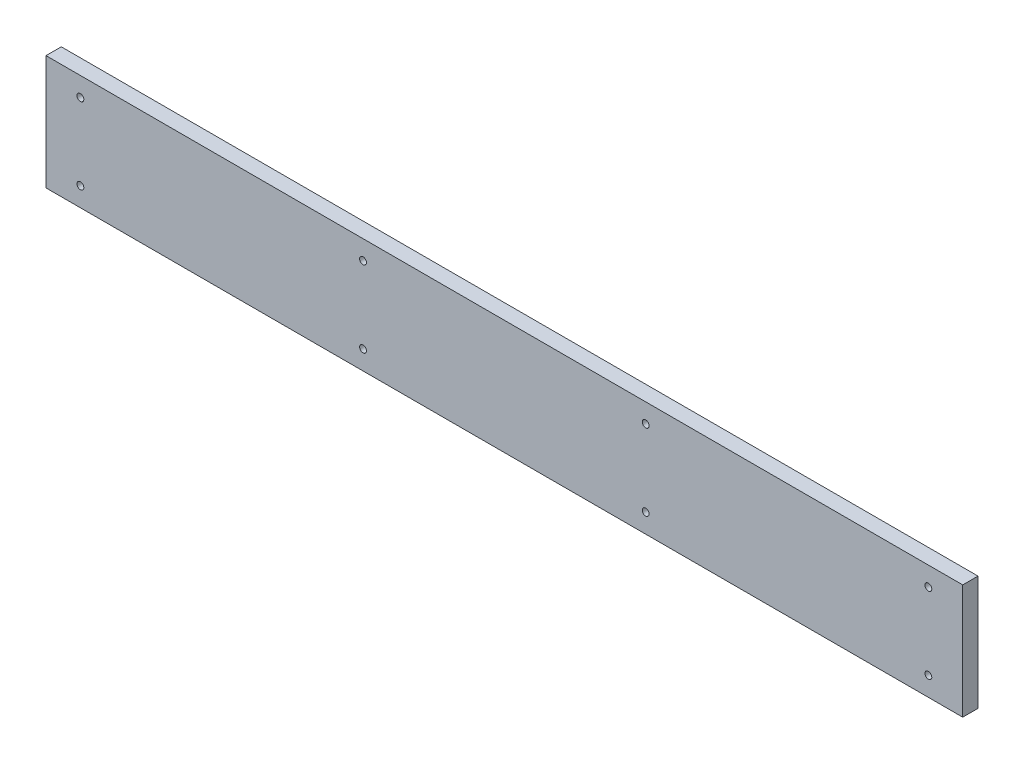
from build123d import *

# Parameters (mm, degrees)
SKETCH1_W                                           = 1200
SKETCH1_H                                           = 150
BOSS_EXTRUDE1_DEPTH                                 = 20
HOLE_SIZE_BY_SOCKET_HEAD_CAP_SCREW_TYPE_D           = 9
HOLE_SIZE_BY_SOCKET_HEAD_CAP_SCREW_TYPE_CBORE_D     = 15
HOLE_SIZE_BY_SOCKET_HEAD_CAP_SCREW_TYPE_CBORE_DEPTH = 9
SKETCH4_R                                           = 22.5
SKETCH4_R_2                                         = 19.5
CUT_EXTRUDE1_DEPTH                                  = 3
LPATTERN1_COUNT                                     = 4
LPATTERN1_PITCH                                     = 30
LPATTERN2_COUNT                                     = 23
LPATTERN2_PITCH                                     = 50
LPATTERN2_COPY_1_SKETCH_R                           = 22.5
LPATTERN2_COPY_1_SKETCH_R_2                         = 19.5
LPATTERN2_COPY_1_DEPTH                              = 3
LPATTERN2_COPY_2_SKETCH_R                           = 22.5
LPATTERN2_COPY_2_SKETCH_R_2                         = 19.5
LPATTERN2_COPY_2_DEPTH                              = 3
LPATTERN2_COPY_3_SKETCH_R                           = 22.5
LPATTERN2_COPY_3_SKETCH_R_2                         = 19.5
LPATTERN2_COPY_3_DEPTH                              = 3
LPATTERN2_COPY_4_SKETCH_R                           = 22.5
LPATTERN2_COPY_4_SKETCH_R_2                         = 19.5
LPATTERN2_COPY_4_DEPTH                              = 3
LPATTERN2_COPY_5_SKETCH_R                           = 22.5
LPATTERN2_COPY_5_SKETCH_R_2                         = 19.5
LPATTERN2_COPY_5_DEPTH                              = 3
LPATTERN2_COPY_6_SKETCH_R                           = 22.5
LPATTERN2_COPY_6_SKETCH_R_2                         = 19.5
LPATTERN2_COPY_6_DEPTH                              = 3
LPATTERN2_COPY_7_SKETCH_R                           = 22.5
LPATTERN2_COPY_7_SKETCH_R_2                         = 19.5
LPATTERN2_COPY_7_DEPTH                              = 3
LPATTERN2_COPY_8_SKETCH_R                           = 22.5
LPATTERN2_COPY_8_SKETCH_R_2                         = 19.5
LPATTERN2_COPY_8_DEPTH                              = 3
LPATTERN2_COPY_9_SKETCH_R                           = 22.5
LPATTERN2_COPY_9_SKETCH_R_2                         = 19.5
LPATTERN2_COPY_9_DEPTH                              = 3
LPATTERN2_COPY_10_SKETCH_R                          = 22.5
LPATTERN2_COPY_10_SKETCH_R_2                        = 19.5
LPATTERN2_COPY_10_DEPTH                             = 3
LPATTERN2_COPY_11_SKETCH_R                          = 22.5
LPATTERN2_COPY_11_SKETCH_R_2                        = 19.5
LPATTERN2_COPY_11_DEPTH                             = 3
LPATTERN2_COPY_12_SKETCH_R                          = 22.5
LPATTERN2_COPY_12_SKETCH_R_2                        = 19.5
LPATTERN2_COPY_12_DEPTH                             = 3
LPATTERN2_COPY_13_SKETCH_R                          = 22.5
LPATTERN2_COPY_13_SKETCH_R_2                        = 19.5
LPATTERN2_COPY_13_DEPTH                             = 3
LPATTERN2_COPY_14_SKETCH_R                          = 22.5
LPATTERN2_COPY_14_SKETCH_R_2                        = 19.5
LPATTERN2_COPY_14_DEPTH                             = 3
LPATTERN2_COPY_15_SKETCH_R                          = 22.5
LPATTERN2_COPY_15_SKETCH_R_2                        = 19.5
LPATTERN2_COPY_15_DEPTH                             = 3
LPATTERN2_COPY_16_SKETCH_R                          = 22.5
LPATTERN2_COPY_16_SKETCH_R_2                        = 19.5
LPATTERN2_COPY_16_DEPTH                             = 3
LPATTERN2_COPY_17_SKETCH_R                          = 22.5
LPATTERN2_COPY_17_SKETCH_R_2                        = 19.5
LPATTERN2_COPY_17_DEPTH                             = 3
LPATTERN2_COPY_18_SKETCH_R                          = 22.5
LPATTERN2_COPY_18_SKETCH_R_2                        = 19.5
LPATTERN2_COPY_18_DEPTH                             = 3
LPATTERN2_COPY_19_SKETCH_R                          = 22.5
LPATTERN2_COPY_19_SKETCH_R_2                        = 19.5
LPATTERN2_COPY_19_DEPTH                             = 3
LPATTERN2_COPY_20_SKETCH_R                          = 22.5
LPATTERN2_COPY_20_SKETCH_R_2                        = 19.5
LPATTERN2_COPY_20_DEPTH                             = 3
LPATTERN2_COPY_21_SKETCH_R                          = 22.5
LPATTERN2_COPY_21_SKETCH_R_2                        = 19.5
LPATTERN2_COPY_21_DEPTH                             = 3
LPATTERN2_COPY_22_SKETCH_R                          = 22.5
LPATTERN2_COPY_22_SKETCH_R_2                        = 19.5
LPATTERN2_COPY_22_DEPTH                             = 3
LPATTERN2_COPY_23_SKETCH_R                          = 22.5
LPATTERN2_COPY_23_SKETCH_R_2                        = 19.5
LPATTERN2_COPY_23_DEPTH                             = 3
LPATTERN2_COPY_24_SKETCH_R                          = 22.5
LPATTERN2_COPY_24_SKETCH_R_2                        = 19.5
LPATTERN2_COPY_24_DEPTH                             = 3
LPATTERN2_COPY_25_SKETCH_R                          = 22.5
LPATTERN2_COPY_25_SKETCH_R_2                        = 19.5
LPATTERN2_COPY_25_DEPTH                             = 3
LPATTERN2_COPY_26_SKETCH_R                          = 22.5
LPATTERN2_COPY_26_SKETCH_R_2                        = 19.5
LPATTERN2_COPY_26_DEPTH                             = 3
LPATTERN2_COPY_27_SKETCH_R                          = 22.5
LPATTERN2_COPY_27_SKETCH_R_2                        = 19.5
LPATTERN2_COPY_27_DEPTH                             = 3
LPATTERN2_COPY_28_SKETCH_R                          = 22.5
LPATTERN2_COPY_28_SKETCH_R_2                        = 19.5
LPATTERN2_COPY_28_DEPTH                             = 3
LPATTERN2_COPY_29_SKETCH_R                          = 22.5
LPATTERN2_COPY_29_SKETCH_R_2                        = 19.5
LPATTERN2_COPY_29_DEPTH                             = 3
LPATTERN2_COPY_30_SKETCH_R                          = 22.5
LPATTERN2_COPY_30_SKETCH_R_2                        = 19.5
LPATTERN2_COPY_30_DEPTH                             = 3
LPATTERN2_COPY_31_SKETCH_R                          = 22.5
LPATTERN2_COPY_31_SKETCH_R_2                        = 19.5
LPATTERN2_COPY_31_DEPTH                             = 3
LPATTERN2_COPY_32_SKETCH_R                          = 22.5
LPATTERN2_COPY_32_SKETCH_R_2                        = 19.5
LPATTERN2_COPY_32_DEPTH                             = 3
LPATTERN2_COPY_33_SKETCH_R                          = 22.5
LPATTERN2_COPY_33_SKETCH_R_2                        = 19.5
LPATTERN2_COPY_33_DEPTH                             = 3
LPATTERN2_COPY_34_SKETCH_R                          = 22.5
LPATTERN2_COPY_34_SKETCH_R_2                        = 19.5
LPATTERN2_COPY_34_DEPTH                             = 3
LPATTERN2_COPY_35_SKETCH_R                          = 22.5
LPATTERN2_COPY_35_SKETCH_R_2                        = 19.5
LPATTERN2_COPY_35_DEPTH                             = 3
LPATTERN2_COPY_36_SKETCH_R                          = 22.5
LPATTERN2_COPY_36_SKETCH_R_2                        = 19.5
LPATTERN2_COPY_36_DEPTH                             = 3
LPATTERN2_COPY_37_SKETCH_R                          = 22.5
LPATTERN2_COPY_37_SKETCH_R_2                        = 19.5
LPATTERN2_COPY_37_DEPTH                             = 3
LPATTERN2_COPY_38_SKETCH_R                          = 22.5
LPATTERN2_COPY_38_SKETCH_R_2                        = 19.5
LPATTERN2_COPY_38_DEPTH                             = 3
LPATTERN2_COPY_39_SKETCH_R                          = 22.5
LPATTERN2_COPY_39_SKETCH_R_2                        = 19.5
LPATTERN2_COPY_39_DEPTH                             = 3
LPATTERN2_COPY_40_SKETCH_R                          = 22.5
LPATTERN2_COPY_40_SKETCH_R_2                        = 19.5
LPATTERN2_COPY_40_DEPTH                             = 3
LPATTERN2_COPY_41_SKETCH_R                          = 22.5
LPATTERN2_COPY_41_SKETCH_R_2                        = 19.5
LPATTERN2_COPY_41_DEPTH                             = 3
LPATTERN2_COPY_42_SKETCH_R                          = 22.5
LPATTERN2_COPY_42_SKETCH_R_2                        = 19.5
LPATTERN2_COPY_42_DEPTH                             = 3
LPATTERN2_COPY_43_SKETCH_R                          = 22.5
LPATTERN2_COPY_43_SKETCH_R_2                        = 19.5
LPATTERN2_COPY_43_DEPTH                             = 3
LPATTERN2_COPY_44_SKETCH_R                          = 22.5
LPATTERN2_COPY_44_SKETCH_R_2                        = 19.5
LPATTERN2_COPY_44_DEPTH                             = 3
LPATTERN2_COPY_45_SKETCH_R                          = 22.5
LPATTERN2_COPY_45_SKETCH_R_2                        = 19.5
LPATTERN2_COPY_45_DEPTH                             = 3
LPATTERN2_COPY_46_SKETCH_R                          = 22.5
LPATTERN2_COPY_46_SKETCH_R_2                        = 19.5
LPATTERN2_COPY_46_DEPTH                             = 3
LPATTERN2_COPY_47_SKETCH_R                          = 22.5
LPATTERN2_COPY_47_SKETCH_R_2                        = 19.5
LPATTERN2_COPY_47_DEPTH                             = 3
LPATTERN2_COPY_48_SKETCH_R                          = 22.5
LPATTERN2_COPY_48_SKETCH_R_2                        = 19.5
LPATTERN2_COPY_48_DEPTH                             = 3
LPATTERN2_COPY_49_SKETCH_R                          = 22.5
LPATTERN2_COPY_49_SKETCH_R_2                        = 19.5
LPATTERN2_COPY_49_DEPTH                             = 3
LPATTERN2_COPY_50_SKETCH_R                          = 22.5
LPATTERN2_COPY_50_SKETCH_R_2                        = 19.5
LPATTERN2_COPY_50_DEPTH                             = 3
LPATTERN2_COPY_51_SKETCH_R                          = 22.5
LPATTERN2_COPY_51_SKETCH_R_2                        = 19.5
LPATTERN2_COPY_51_DEPTH                             = 3
LPATTERN2_COPY_52_SKETCH_R                          = 22.5
LPATTERN2_COPY_52_SKETCH_R_2                        = 19.5
LPATTERN2_COPY_52_DEPTH                             = 3
LPATTERN2_COPY_53_SKETCH_R                          = 22.5
LPATTERN2_COPY_53_SKETCH_R_2                        = 19.5
LPATTERN2_COPY_53_DEPTH                             = 3
LPATTERN2_COPY_54_SKETCH_R                          = 22.5
LPATTERN2_COPY_54_SKETCH_R_2                        = 19.5
LPATTERN2_COPY_54_DEPTH                             = 3
LPATTERN2_COPY_55_SKETCH_R                          = 22.5
LPATTERN2_COPY_55_SKETCH_R_2                        = 19.5
LPATTERN2_COPY_55_DEPTH                             = 3
LPATTERN2_COPY_56_SKETCH_R                          = 22.5
LPATTERN2_COPY_56_SKETCH_R_2                        = 19.5
LPATTERN2_COPY_56_DEPTH                             = 3
LPATTERN2_COPY_57_SKETCH_R                          = 22.5
LPATTERN2_COPY_57_SKETCH_R_2                        = 19.5
LPATTERN2_COPY_57_DEPTH                             = 3
LPATTERN2_COPY_58_SKETCH_R                          = 22.5
LPATTERN2_COPY_58_SKETCH_R_2                        = 19.5
LPATTERN2_COPY_58_DEPTH                             = 3
LPATTERN2_COPY_59_SKETCH_R                          = 22.5
LPATTERN2_COPY_59_SKETCH_R_2                        = 19.5
LPATTERN2_COPY_59_DEPTH                             = 3
LPATTERN2_COPY_60_SKETCH_R                          = 22.5
LPATTERN2_COPY_60_SKETCH_R_2                        = 19.5
LPATTERN2_COPY_60_DEPTH                             = 3
LPATTERN2_COPY_61_SKETCH_R                          = 22.5
LPATTERN2_COPY_61_SKETCH_R_2                        = 19.5
LPATTERN2_COPY_61_DEPTH                             = 3
LPATTERN2_COPY_62_SKETCH_R                          = 22.5
LPATTERN2_COPY_62_SKETCH_R_2                        = 19.5
LPATTERN2_COPY_62_DEPTH                             = 3
LPATTERN2_COPY_63_SKETCH_R                          = 22.5
LPATTERN2_COPY_63_SKETCH_R_2                        = 19.5
LPATTERN2_COPY_63_DEPTH                             = 3
LPATTERN2_COPY_64_SKETCH_R                          = 22.5
LPATTERN2_COPY_64_SKETCH_R_2                        = 19.5
LPATTERN2_COPY_64_DEPTH                             = 3
LPATTERN2_COPY_65_SKETCH_R                          = 22.5
LPATTERN2_COPY_65_SKETCH_R_2                        = 19.5
LPATTERN2_COPY_65_DEPTH                             = 3
LPATTERN2_COPY_66_SKETCH_R                          = 22.5
LPATTERN2_COPY_66_SKETCH_R_2                        = 19.5
LPATTERN2_COPY_66_DEPTH                             = 3


with BuildPart() as part:
    # Sketch1 → Boss-Extrude1 (new body)
    with BuildSketch(Plane.XY):
        with Locations((600, 75)):
            Rectangle(SKETCH1_W, SKETCH1_H)
    extrude(amount=BOSS_EXTRUDE1_DEPTH)

    # Hole size (by socket head cap screw type)1 (through all)
    with Locations(Plane(origin=(0, 0, 0), x_dir=(-1, 0, 0), z_dir=(0, 0, -1))):
        with Locations((-1155, 125), (-1155, 25), (-785, 25), (-415, 25), (-45, 25), (-45, 125), (-415, 125), (-785, 125)):
            CounterBoreHole(HOLE_SIZE_BY_SOCKET_HEAD_CAP_SCREW_TYPE_D / 2, HOLE_SIZE_BY_SOCKET_HEAD_CAP_SCREW_TYPE_CBORE_D / 2, HOLE_SIZE_BY_SOCKET_HEAD_CAP_SCREW_TYPE_CBORE_DEPTH)

    # Sketch4 → Cut-Extrude1 (cut)
    with BuildSketch(Plane(origin=(0, 0, 0), x_dir=(-1, 0, 0), z_dir=(0, 0, -1))):
        with Locations((-50, 30)):
            Circle(SKETCH4_R)
        with Locations((-50, 30)):
            Circle(SKETCH4_R_2, mode=Mode.SUBTRACT)
    cut_extrude1 = extrude(amount=-CUT_EXTRUDE1_DEPTH, mode=Mode.SUBTRACT)

    # LPattern1: Cut-Extrude1 ×4
    with Locations(*[(0, i * LPATTERN1_PITCH, 0) for i in range(1, LPATTERN1_COUNT)]):
        add(cut_extrude1, mode=Mode.SUBTRACT)

    # LPattern2: Cut-Extrude1 ×23
    with Locations(*[(i * LPATTERN2_PITCH, 0, 0) for i in range(1, LPATTERN2_COUNT)]):
        add(cut_extrude1, mode=Mode.SUBTRACT)

    # LPattern2 copy 1 sketch → LPattern2 copy 1 (cut)
    with BuildSketch(Plane(origin=(50, 30, 0), x_dir=(-1, 0, 0), z_dir=(0, 0, -1))):
        with Locations((-50, 30)):
            Circle(LPATTERN2_COPY_1_SKETCH_R)
        with Locations((-50, 30)):
            Circle(LPATTERN2_COPY_1_SKETCH_R_2, mode=Mode.SUBTRACT)
    extrude(amount=-LPATTERN2_COPY_1_DEPTH, mode=Mode.SUBTRACT)

    # LPattern2 copy 2 sketch → LPattern2 copy 2 (cut)
    with BuildSketch(Plane(origin=(100, 30, 0), x_dir=(-1, 0, 0), z_dir=(0, 0, -1))):
        with Locations((-50, 30)):
            Circle(LPATTERN2_COPY_2_SKETCH_R)
        with Locations((-50, 30)):
            Circle(LPATTERN2_COPY_2_SKETCH_R_2, mode=Mode.SUBTRACT)
    extrude(amount=-LPATTERN2_COPY_2_DEPTH, mode=Mode.SUBTRACT)

    # LPattern2 copy 3 sketch → LPattern2 copy 3 (cut)
    with BuildSketch(Plane(origin=(150, 30, 0), x_dir=(-1, 0, 0), z_dir=(0, 0, -1))):
        with Locations((-50, 30)):
            Circle(LPATTERN2_COPY_3_SKETCH_R)
        with Locations((-50, 30)):
            Circle(LPATTERN2_COPY_3_SKETCH_R_2, mode=Mode.SUBTRACT)
    extrude(amount=-LPATTERN2_COPY_3_DEPTH, mode=Mode.SUBTRACT)

    # LPattern2 copy 4 sketch → LPattern2 copy 4 (cut)
    with BuildSketch(Plane(origin=(200, 30, 0), x_dir=(-1, 0, 0), z_dir=(0, 0, -1))):
        with Locations((-50, 30)):
            Circle(LPATTERN2_COPY_4_SKETCH_R)
        with Locations((-50, 30)):
            Circle(LPATTERN2_COPY_4_SKETCH_R_2, mode=Mode.SUBTRACT)
    extrude(amount=-LPATTERN2_COPY_4_DEPTH, mode=Mode.SUBTRACT)

    # LPattern2 copy 5 sketch → LPattern2 copy 5 (cut)
    with BuildSketch(Plane(origin=(250, 30, 0), x_dir=(-1, 0, 0), z_dir=(0, 0, -1))):
        with Locations((-50, 30)):
            Circle(LPATTERN2_COPY_5_SKETCH_R)
        with Locations((-50, 30)):
            Circle(LPATTERN2_COPY_5_SKETCH_R_2, mode=Mode.SUBTRACT)
    extrude(amount=-LPATTERN2_COPY_5_DEPTH, mode=Mode.SUBTRACT)

    # LPattern2 copy 6 sketch → LPattern2 copy 6 (cut)
    with BuildSketch(Plane(origin=(300, 30, 0), x_dir=(-1, 0, 0), z_dir=(0, 0, -1))):
        with Locations((-50, 30)):
            Circle(LPATTERN2_COPY_6_SKETCH_R)
        with Locations((-50, 30)):
            Circle(LPATTERN2_COPY_6_SKETCH_R_2, mode=Mode.SUBTRACT)
    extrude(amount=-LPATTERN2_COPY_6_DEPTH, mode=Mode.SUBTRACT)

    # LPattern2 copy 7 sketch → LPattern2 copy 7 (cut)
    with BuildSketch(Plane(origin=(350, 30, 0), x_dir=(-1, 0, 0), z_dir=(0, 0, -1))):
        with Locations((-50, 30)):
            Circle(LPATTERN2_COPY_7_SKETCH_R)
        with Locations((-50, 30)):
            Circle(LPATTERN2_COPY_7_SKETCH_R_2, mode=Mode.SUBTRACT)
    extrude(amount=-LPATTERN2_COPY_7_DEPTH, mode=Mode.SUBTRACT)

    # LPattern2 copy 8 sketch → LPattern2 copy 8 (cut)
    with BuildSketch(Plane(origin=(400, 30, 0), x_dir=(-1, 0, 0), z_dir=(0, 0, -1))):
        with Locations((-50, 30)):
            Circle(LPATTERN2_COPY_8_SKETCH_R)
        with Locations((-50, 30)):
            Circle(LPATTERN2_COPY_8_SKETCH_R_2, mode=Mode.SUBTRACT)
    extrude(amount=-LPATTERN2_COPY_8_DEPTH, mode=Mode.SUBTRACT)

    # LPattern2 copy 9 sketch → LPattern2 copy 9 (cut)
    with BuildSketch(Plane(origin=(450, 30, 0), x_dir=(-1, 0, 0), z_dir=(0, 0, -1))):
        with Locations((-50, 30)):
            Circle(LPATTERN2_COPY_9_SKETCH_R)
        with Locations((-50, 30)):
            Circle(LPATTERN2_COPY_9_SKETCH_R_2, mode=Mode.SUBTRACT)
    extrude(amount=-LPATTERN2_COPY_9_DEPTH, mode=Mode.SUBTRACT)

    # LPattern2 copy 10 sketch → LPattern2 copy 10 (cut)
    with BuildSketch(Plane(origin=(500, 30, 0), x_dir=(-1, 0, 0), z_dir=(0, 0, -1))):
        with Locations((-50, 30)):
            Circle(LPATTERN2_COPY_10_SKETCH_R)
        with Locations((-50, 30)):
            Circle(LPATTERN2_COPY_10_SKETCH_R_2, mode=Mode.SUBTRACT)
    extrude(amount=-LPATTERN2_COPY_10_DEPTH, mode=Mode.SUBTRACT)

    # LPattern2 copy 11 sketch → LPattern2 copy 11 (cut)
    with BuildSketch(Plane(origin=(550, 30, 0), x_dir=(-1, 0, 0), z_dir=(0, 0, -1))):
        with Locations((-50, 30)):
            Circle(LPATTERN2_COPY_11_SKETCH_R)
        with Locations((-50, 30)):
            Circle(LPATTERN2_COPY_11_SKETCH_R_2, mode=Mode.SUBTRACT)
    extrude(amount=-LPATTERN2_COPY_11_DEPTH, mode=Mode.SUBTRACT)

    # LPattern2 copy 12 sketch → LPattern2 copy 12 (cut)
    with BuildSketch(Plane(origin=(600, 30, 0), x_dir=(-1, 0, 0), z_dir=(0, 0, -1))):
        with Locations((-50, 30)):
            Circle(LPATTERN2_COPY_12_SKETCH_R)
        with Locations((-50, 30)):
            Circle(LPATTERN2_COPY_12_SKETCH_R_2, mode=Mode.SUBTRACT)
    extrude(amount=-LPATTERN2_COPY_12_DEPTH, mode=Mode.SUBTRACT)

    # LPattern2 copy 13 sketch → LPattern2 copy 13 (cut)
    with BuildSketch(Plane(origin=(650, 30, 0), x_dir=(-1, 0, 0), z_dir=(0, 0, -1))):
        with Locations((-50, 30)):
            Circle(LPATTERN2_COPY_13_SKETCH_R)
        with Locations((-50, 30)):
            Circle(LPATTERN2_COPY_13_SKETCH_R_2, mode=Mode.SUBTRACT)
    extrude(amount=-LPATTERN2_COPY_13_DEPTH, mode=Mode.SUBTRACT)

    # LPattern2 copy 14 sketch → LPattern2 copy 14 (cut)
    with BuildSketch(Plane(origin=(700, 30, 0), x_dir=(-1, 0, 0), z_dir=(0, 0, -1))):
        with Locations((-50, 30)):
            Circle(LPATTERN2_COPY_14_SKETCH_R)
        with Locations((-50, 30)):
            Circle(LPATTERN2_COPY_14_SKETCH_R_2, mode=Mode.SUBTRACT)
    extrude(amount=-LPATTERN2_COPY_14_DEPTH, mode=Mode.SUBTRACT)

    # LPattern2 copy 15 sketch → LPattern2 copy 15 (cut)
    with BuildSketch(Plane(origin=(750, 30, 0), x_dir=(-1, 0, 0), z_dir=(0, 0, -1))):
        with Locations((-50, 30)):
            Circle(LPATTERN2_COPY_15_SKETCH_R)
        with Locations((-50, 30)):
            Circle(LPATTERN2_COPY_15_SKETCH_R_2, mode=Mode.SUBTRACT)
    extrude(amount=-LPATTERN2_COPY_15_DEPTH, mode=Mode.SUBTRACT)

    # LPattern2 copy 16 sketch → LPattern2 copy 16 (cut)
    with BuildSketch(Plane(origin=(800, 30, 0), x_dir=(-1, 0, 0), z_dir=(0, 0, -1))):
        with Locations((-50, 30)):
            Circle(LPATTERN2_COPY_16_SKETCH_R)
        with Locations((-50, 30)):
            Circle(LPATTERN2_COPY_16_SKETCH_R_2, mode=Mode.SUBTRACT)
    extrude(amount=-LPATTERN2_COPY_16_DEPTH, mode=Mode.SUBTRACT)

    # LPattern2 copy 17 sketch → LPattern2 copy 17 (cut)
    with BuildSketch(Plane(origin=(850, 30, 0), x_dir=(-1, 0, 0), z_dir=(0, 0, -1))):
        with Locations((-50, 30)):
            Circle(LPATTERN2_COPY_17_SKETCH_R)
        with Locations((-50, 30)):
            Circle(LPATTERN2_COPY_17_SKETCH_R_2, mode=Mode.SUBTRACT)
    extrude(amount=-LPATTERN2_COPY_17_DEPTH, mode=Mode.SUBTRACT)

    # LPattern2 copy 18 sketch → LPattern2 copy 18 (cut)
    with BuildSketch(Plane(origin=(900, 30, 0), x_dir=(-1, 0, 0), z_dir=(0, 0, -1))):
        with Locations((-50, 30)):
            Circle(LPATTERN2_COPY_18_SKETCH_R)
        with Locations((-50, 30)):
            Circle(LPATTERN2_COPY_18_SKETCH_R_2, mode=Mode.SUBTRACT)
    extrude(amount=-LPATTERN2_COPY_18_DEPTH, mode=Mode.SUBTRACT)

    # LPattern2 copy 19 sketch → LPattern2 copy 19 (cut)
    with BuildSketch(Plane(origin=(950, 30, 0), x_dir=(-1, 0, 0), z_dir=(0, 0, -1))):
        with Locations((-50, 30)):
            Circle(LPATTERN2_COPY_19_SKETCH_R)
        with Locations((-50, 30)):
            Circle(LPATTERN2_COPY_19_SKETCH_R_2, mode=Mode.SUBTRACT)
    extrude(amount=-LPATTERN2_COPY_19_DEPTH, mode=Mode.SUBTRACT)

    # LPattern2 copy 20 sketch → LPattern2 copy 20 (cut)
    with BuildSketch(Plane(origin=(1000, 30, 0), x_dir=(-1, 0, 0), z_dir=(0, 0, -1))):
        with Locations((-50, 30)):
            Circle(LPATTERN2_COPY_20_SKETCH_R)
        with Locations((-50, 30)):
            Circle(LPATTERN2_COPY_20_SKETCH_R_2, mode=Mode.SUBTRACT)
    extrude(amount=-LPATTERN2_COPY_20_DEPTH, mode=Mode.SUBTRACT)

    # LPattern2 copy 21 sketch → LPattern2 copy 21 (cut)
    with BuildSketch(Plane(origin=(1050, 30, 0), x_dir=(-1, 0, 0), z_dir=(0, 0, -1))):
        with Locations((-50, 30)):
            Circle(LPATTERN2_COPY_21_SKETCH_R)
        with Locations((-50, 30)):
            Circle(LPATTERN2_COPY_21_SKETCH_R_2, mode=Mode.SUBTRACT)
    extrude(amount=-LPATTERN2_COPY_21_DEPTH, mode=Mode.SUBTRACT)

    # LPattern2 copy 22 sketch → LPattern2 copy 22 (cut)
    with BuildSketch(Plane(origin=(1100, 30, 0), x_dir=(-1, 0, 0), z_dir=(0, 0, -1))):
        with Locations((-50, 30)):
            Circle(LPATTERN2_COPY_22_SKETCH_R)
        with Locations((-50, 30)):
            Circle(LPATTERN2_COPY_22_SKETCH_R_2, mode=Mode.SUBTRACT)
    extrude(amount=-LPATTERN2_COPY_22_DEPTH, mode=Mode.SUBTRACT)

    # LPattern2 copy 23 sketch → LPattern2 copy 23 (cut)
    with BuildSketch(Plane(origin=(50, 60, 0), x_dir=(-1, 0, 0), z_dir=(0, 0, -1))):
        with Locations((-50, 30)):
            Circle(LPATTERN2_COPY_23_SKETCH_R)
        with Locations((-50, 30)):
            Circle(LPATTERN2_COPY_23_SKETCH_R_2, mode=Mode.SUBTRACT)
    extrude(amount=-LPATTERN2_COPY_23_DEPTH, mode=Mode.SUBTRACT)

    # LPattern2 copy 24 sketch → LPattern2 copy 24 (cut)
    with BuildSketch(Plane(origin=(100, 60, 0), x_dir=(-1, 0, 0), z_dir=(0, 0, -1))):
        with Locations((-50, 30)):
            Circle(LPATTERN2_COPY_24_SKETCH_R)
        with Locations((-50, 30)):
            Circle(LPATTERN2_COPY_24_SKETCH_R_2, mode=Mode.SUBTRACT)
    extrude(amount=-LPATTERN2_COPY_24_DEPTH, mode=Mode.SUBTRACT)

    # LPattern2 copy 25 sketch → LPattern2 copy 25 (cut)
    with BuildSketch(Plane(origin=(150, 60, 0), x_dir=(-1, 0, 0), z_dir=(0, 0, -1))):
        with Locations((-50, 30)):
            Circle(LPATTERN2_COPY_25_SKETCH_R)
        with Locations((-50, 30)):
            Circle(LPATTERN2_COPY_25_SKETCH_R_2, mode=Mode.SUBTRACT)
    extrude(amount=-LPATTERN2_COPY_25_DEPTH, mode=Mode.SUBTRACT)

    # LPattern2 copy 26 sketch → LPattern2 copy 26 (cut)
    with BuildSketch(Plane(origin=(200, 60, 0), x_dir=(-1, 0, 0), z_dir=(0, 0, -1))):
        with Locations((-50, 30)):
            Circle(LPATTERN2_COPY_26_SKETCH_R)
        with Locations((-50, 30)):
            Circle(LPATTERN2_COPY_26_SKETCH_R_2, mode=Mode.SUBTRACT)
    extrude(amount=-LPATTERN2_COPY_26_DEPTH, mode=Mode.SUBTRACT)

    # LPattern2 copy 27 sketch → LPattern2 copy 27 (cut)
    with BuildSketch(Plane(origin=(250, 60, 0), x_dir=(-1, 0, 0), z_dir=(0, 0, -1))):
        with Locations((-50, 30)):
            Circle(LPATTERN2_COPY_27_SKETCH_R)
        with Locations((-50, 30)):
            Circle(LPATTERN2_COPY_27_SKETCH_R_2, mode=Mode.SUBTRACT)
    extrude(amount=-LPATTERN2_COPY_27_DEPTH, mode=Mode.SUBTRACT)

    # LPattern2 copy 28 sketch → LPattern2 copy 28 (cut)
    with BuildSketch(Plane(origin=(300, 60, 0), x_dir=(-1, 0, 0), z_dir=(0, 0, -1))):
        with Locations((-50, 30)):
            Circle(LPATTERN2_COPY_28_SKETCH_R)
        with Locations((-50, 30)):
            Circle(LPATTERN2_COPY_28_SKETCH_R_2, mode=Mode.SUBTRACT)
    extrude(amount=-LPATTERN2_COPY_28_DEPTH, mode=Mode.SUBTRACT)

    # LPattern2 copy 29 sketch → LPattern2 copy 29 (cut)
    with BuildSketch(Plane(origin=(350, 60, 0), x_dir=(-1, 0, 0), z_dir=(0, 0, -1))):
        with Locations((-50, 30)):
            Circle(LPATTERN2_COPY_29_SKETCH_R)
        with Locations((-50, 30)):
            Circle(LPATTERN2_COPY_29_SKETCH_R_2, mode=Mode.SUBTRACT)
    extrude(amount=-LPATTERN2_COPY_29_DEPTH, mode=Mode.SUBTRACT)

    # LPattern2 copy 30 sketch → LPattern2 copy 30 (cut)
    with BuildSketch(Plane(origin=(400, 60, 0), x_dir=(-1, 0, 0), z_dir=(0, 0, -1))):
        with Locations((-50, 30)):
            Circle(LPATTERN2_COPY_30_SKETCH_R)
        with Locations((-50, 30)):
            Circle(LPATTERN2_COPY_30_SKETCH_R_2, mode=Mode.SUBTRACT)
    extrude(amount=-LPATTERN2_COPY_30_DEPTH, mode=Mode.SUBTRACT)

    # LPattern2 copy 31 sketch → LPattern2 copy 31 (cut)
    with BuildSketch(Plane(origin=(450, 60, 0), x_dir=(-1, 0, 0), z_dir=(0, 0, -1))):
        with Locations((-50, 30)):
            Circle(LPATTERN2_COPY_31_SKETCH_R)
        with Locations((-50, 30)):
            Circle(LPATTERN2_COPY_31_SKETCH_R_2, mode=Mode.SUBTRACT)
    extrude(amount=-LPATTERN2_COPY_31_DEPTH, mode=Mode.SUBTRACT)

    # LPattern2 copy 32 sketch → LPattern2 copy 32 (cut)
    with BuildSketch(Plane(origin=(500, 60, 0), x_dir=(-1, 0, 0), z_dir=(0, 0, -1))):
        with Locations((-50, 30)):
            Circle(LPATTERN2_COPY_32_SKETCH_R)
        with Locations((-50, 30)):
            Circle(LPATTERN2_COPY_32_SKETCH_R_2, mode=Mode.SUBTRACT)
    extrude(amount=-LPATTERN2_COPY_32_DEPTH, mode=Mode.SUBTRACT)

    # LPattern2 copy 33 sketch → LPattern2 copy 33 (cut)
    with BuildSketch(Plane(origin=(550, 60, 0), x_dir=(-1, 0, 0), z_dir=(0, 0, -1))):
        with Locations((-50, 30)):
            Circle(LPATTERN2_COPY_33_SKETCH_R)
        with Locations((-50, 30)):
            Circle(LPATTERN2_COPY_33_SKETCH_R_2, mode=Mode.SUBTRACT)
    extrude(amount=-LPATTERN2_COPY_33_DEPTH, mode=Mode.SUBTRACT)

    # LPattern2 copy 34 sketch → LPattern2 copy 34 (cut)
    with BuildSketch(Plane(origin=(600, 60, 0), x_dir=(-1, 0, 0), z_dir=(0, 0, -1))):
        with Locations((-50, 30)):
            Circle(LPATTERN2_COPY_34_SKETCH_R)
        with Locations((-50, 30)):
            Circle(LPATTERN2_COPY_34_SKETCH_R_2, mode=Mode.SUBTRACT)
    extrude(amount=-LPATTERN2_COPY_34_DEPTH, mode=Mode.SUBTRACT)

    # LPattern2 copy 35 sketch → LPattern2 copy 35 (cut)
    with BuildSketch(Plane(origin=(650, 60, 0), x_dir=(-1, 0, 0), z_dir=(0, 0, -1))):
        with Locations((-50, 30)):
            Circle(LPATTERN2_COPY_35_SKETCH_R)
        with Locations((-50, 30)):
            Circle(LPATTERN2_COPY_35_SKETCH_R_2, mode=Mode.SUBTRACT)
    extrude(amount=-LPATTERN2_COPY_35_DEPTH, mode=Mode.SUBTRACT)

    # LPattern2 copy 36 sketch → LPattern2 copy 36 (cut)
    with BuildSketch(Plane(origin=(700, 60, 0), x_dir=(-1, 0, 0), z_dir=(0, 0, -1))):
        with Locations((-50, 30)):
            Circle(LPATTERN2_COPY_36_SKETCH_R)
        with Locations((-50, 30)):
            Circle(LPATTERN2_COPY_36_SKETCH_R_2, mode=Mode.SUBTRACT)
    extrude(amount=-LPATTERN2_COPY_36_DEPTH, mode=Mode.SUBTRACT)

    # LPattern2 copy 37 sketch → LPattern2 copy 37 (cut)
    with BuildSketch(Plane(origin=(750, 60, 0), x_dir=(-1, 0, 0), z_dir=(0, 0, -1))):
        with Locations((-50, 30)):
            Circle(LPATTERN2_COPY_37_SKETCH_R)
        with Locations((-50, 30)):
            Circle(LPATTERN2_COPY_37_SKETCH_R_2, mode=Mode.SUBTRACT)
    extrude(amount=-LPATTERN2_COPY_37_DEPTH, mode=Mode.SUBTRACT)

    # LPattern2 copy 38 sketch → LPattern2 copy 38 (cut)
    with BuildSketch(Plane(origin=(800, 60, 0), x_dir=(-1, 0, 0), z_dir=(0, 0, -1))):
        with Locations((-50, 30)):
            Circle(LPATTERN2_COPY_38_SKETCH_R)
        with Locations((-50, 30)):
            Circle(LPATTERN2_COPY_38_SKETCH_R_2, mode=Mode.SUBTRACT)
    extrude(amount=-LPATTERN2_COPY_38_DEPTH, mode=Mode.SUBTRACT)

    # LPattern2 copy 39 sketch → LPattern2 copy 39 (cut)
    with BuildSketch(Plane(origin=(850, 60, 0), x_dir=(-1, 0, 0), z_dir=(0, 0, -1))):
        with Locations((-50, 30)):
            Circle(LPATTERN2_COPY_39_SKETCH_R)
        with Locations((-50, 30)):
            Circle(LPATTERN2_COPY_39_SKETCH_R_2, mode=Mode.SUBTRACT)
    extrude(amount=-LPATTERN2_COPY_39_DEPTH, mode=Mode.SUBTRACT)

    # LPattern2 copy 40 sketch → LPattern2 copy 40 (cut)
    with BuildSketch(Plane(origin=(900, 60, 0), x_dir=(-1, 0, 0), z_dir=(0, 0, -1))):
        with Locations((-50, 30)):
            Circle(LPATTERN2_COPY_40_SKETCH_R)
        with Locations((-50, 30)):
            Circle(LPATTERN2_COPY_40_SKETCH_R_2, mode=Mode.SUBTRACT)
    extrude(amount=-LPATTERN2_COPY_40_DEPTH, mode=Mode.SUBTRACT)

    # LPattern2 copy 41 sketch → LPattern2 copy 41 (cut)
    with BuildSketch(Plane(origin=(950, 60, 0), x_dir=(-1, 0, 0), z_dir=(0, 0, -1))):
        with Locations((-50, 30)):
            Circle(LPATTERN2_COPY_41_SKETCH_R)
        with Locations((-50, 30)):
            Circle(LPATTERN2_COPY_41_SKETCH_R_2, mode=Mode.SUBTRACT)
    extrude(amount=-LPATTERN2_COPY_41_DEPTH, mode=Mode.SUBTRACT)

    # LPattern2 copy 42 sketch → LPattern2 copy 42 (cut)
    with BuildSketch(Plane(origin=(1000, 60, 0), x_dir=(-1, 0, 0), z_dir=(0, 0, -1))):
        with Locations((-50, 30)):
            Circle(LPATTERN2_COPY_42_SKETCH_R)
        with Locations((-50, 30)):
            Circle(LPATTERN2_COPY_42_SKETCH_R_2, mode=Mode.SUBTRACT)
    extrude(amount=-LPATTERN2_COPY_42_DEPTH, mode=Mode.SUBTRACT)

    # LPattern2 copy 43 sketch → LPattern2 copy 43 (cut)
    with BuildSketch(Plane(origin=(1050, 60, 0), x_dir=(-1, 0, 0), z_dir=(0, 0, -1))):
        with Locations((-50, 30)):
            Circle(LPATTERN2_COPY_43_SKETCH_R)
        with Locations((-50, 30)):
            Circle(LPATTERN2_COPY_43_SKETCH_R_2, mode=Mode.SUBTRACT)
    extrude(amount=-LPATTERN2_COPY_43_DEPTH, mode=Mode.SUBTRACT)

    # LPattern2 copy 44 sketch → LPattern2 copy 44 (cut)
    with BuildSketch(Plane(origin=(1100, 60, 0), x_dir=(-1, 0, 0), z_dir=(0, 0, -1))):
        with Locations((-50, 30)):
            Circle(LPATTERN2_COPY_44_SKETCH_R)
        with Locations((-50, 30)):
            Circle(LPATTERN2_COPY_44_SKETCH_R_2, mode=Mode.SUBTRACT)
    extrude(amount=-LPATTERN2_COPY_44_DEPTH, mode=Mode.SUBTRACT)

    # LPattern2 copy 45 sketch → LPattern2 copy 45 (cut)
    with BuildSketch(Plane(origin=(50, 90, 0), x_dir=(-1, 0, 0), z_dir=(0, 0, -1))):
        with Locations((-50, 30)):
            Circle(LPATTERN2_COPY_45_SKETCH_R)
        with Locations((-50, 30)):
            Circle(LPATTERN2_COPY_45_SKETCH_R_2, mode=Mode.SUBTRACT)
    extrude(amount=-LPATTERN2_COPY_45_DEPTH, mode=Mode.SUBTRACT)

    # LPattern2 copy 46 sketch → LPattern2 copy 46 (cut)
    with BuildSketch(Plane(origin=(100, 90, 0), x_dir=(-1, 0, 0), z_dir=(0, 0, -1))):
        with Locations((-50, 30)):
            Circle(LPATTERN2_COPY_46_SKETCH_R)
        with Locations((-50, 30)):
            Circle(LPATTERN2_COPY_46_SKETCH_R_2, mode=Mode.SUBTRACT)
    extrude(amount=-LPATTERN2_COPY_46_DEPTH, mode=Mode.SUBTRACT)

    # LPattern2 copy 47 sketch → LPattern2 copy 47 (cut)
    with BuildSketch(Plane(origin=(150, 90, 0), x_dir=(-1, 0, 0), z_dir=(0, 0, -1))):
        with Locations((-50, 30)):
            Circle(LPATTERN2_COPY_47_SKETCH_R)
        with Locations((-50, 30)):
            Circle(LPATTERN2_COPY_47_SKETCH_R_2, mode=Mode.SUBTRACT)
    extrude(amount=-LPATTERN2_COPY_47_DEPTH, mode=Mode.SUBTRACT)

    # LPattern2 copy 48 sketch → LPattern2 copy 48 (cut)
    with BuildSketch(Plane(origin=(200, 90, 0), x_dir=(-1, 0, 0), z_dir=(0, 0, -1))):
        with Locations((-50, 30)):
            Circle(LPATTERN2_COPY_48_SKETCH_R)
        with Locations((-50, 30)):
            Circle(LPATTERN2_COPY_48_SKETCH_R_2, mode=Mode.SUBTRACT)
    extrude(amount=-LPATTERN2_COPY_48_DEPTH, mode=Mode.SUBTRACT)

    # LPattern2 copy 49 sketch → LPattern2 copy 49 (cut)
    with BuildSketch(Plane(origin=(250, 90, 0), x_dir=(-1, 0, 0), z_dir=(0, 0, -1))):
        with Locations((-50, 30)):
            Circle(LPATTERN2_COPY_49_SKETCH_R)
        with Locations((-50, 30)):
            Circle(LPATTERN2_COPY_49_SKETCH_R_2, mode=Mode.SUBTRACT)
    extrude(amount=-LPATTERN2_COPY_49_DEPTH, mode=Mode.SUBTRACT)

    # LPattern2 copy 50 sketch → LPattern2 copy 50 (cut)
    with BuildSketch(Plane(origin=(300, 90, 0), x_dir=(-1, 0, 0), z_dir=(0, 0, -1))):
        with Locations((-50, 30)):
            Circle(LPATTERN2_COPY_50_SKETCH_R)
        with Locations((-50, 30)):
            Circle(LPATTERN2_COPY_50_SKETCH_R_2, mode=Mode.SUBTRACT)
    extrude(amount=-LPATTERN2_COPY_50_DEPTH, mode=Mode.SUBTRACT)

    # LPattern2 copy 51 sketch → LPattern2 copy 51 (cut)
    with BuildSketch(Plane(origin=(350, 90, 0), x_dir=(-1, 0, 0), z_dir=(0, 0, -1))):
        with Locations((-50, 30)):
            Circle(LPATTERN2_COPY_51_SKETCH_R)
        with Locations((-50, 30)):
            Circle(LPATTERN2_COPY_51_SKETCH_R_2, mode=Mode.SUBTRACT)
    extrude(amount=-LPATTERN2_COPY_51_DEPTH, mode=Mode.SUBTRACT)

    # LPattern2 copy 52 sketch → LPattern2 copy 52 (cut)
    with BuildSketch(Plane(origin=(400, 90, 0), x_dir=(-1, 0, 0), z_dir=(0, 0, -1))):
        with Locations((-50, 30)):
            Circle(LPATTERN2_COPY_52_SKETCH_R)
        with Locations((-50, 30)):
            Circle(LPATTERN2_COPY_52_SKETCH_R_2, mode=Mode.SUBTRACT)
    extrude(amount=-LPATTERN2_COPY_52_DEPTH, mode=Mode.SUBTRACT)

    # LPattern2 copy 53 sketch → LPattern2 copy 53 (cut)
    with BuildSketch(Plane(origin=(450, 90, 0), x_dir=(-1, 0, 0), z_dir=(0, 0, -1))):
        with Locations((-50, 30)):
            Circle(LPATTERN2_COPY_53_SKETCH_R)
        with Locations((-50, 30)):
            Circle(LPATTERN2_COPY_53_SKETCH_R_2, mode=Mode.SUBTRACT)
    extrude(amount=-LPATTERN2_COPY_53_DEPTH, mode=Mode.SUBTRACT)

    # LPattern2 copy 54 sketch → LPattern2 copy 54 (cut)
    with BuildSketch(Plane(origin=(500, 90, 0), x_dir=(-1, 0, 0), z_dir=(0, 0, -1))):
        with Locations((-50, 30)):
            Circle(LPATTERN2_COPY_54_SKETCH_R)
        with Locations((-50, 30)):
            Circle(LPATTERN2_COPY_54_SKETCH_R_2, mode=Mode.SUBTRACT)
    extrude(amount=-LPATTERN2_COPY_54_DEPTH, mode=Mode.SUBTRACT)

    # LPattern2 copy 55 sketch → LPattern2 copy 55 (cut)
    with BuildSketch(Plane(origin=(550, 90, 0), x_dir=(-1, 0, 0), z_dir=(0, 0, -1))):
        with Locations((-50, 30)):
            Circle(LPATTERN2_COPY_55_SKETCH_R)
        with Locations((-50, 30)):
            Circle(LPATTERN2_COPY_55_SKETCH_R_2, mode=Mode.SUBTRACT)
    extrude(amount=-LPATTERN2_COPY_55_DEPTH, mode=Mode.SUBTRACT)

    # LPattern2 copy 56 sketch → LPattern2 copy 56 (cut)
    with BuildSketch(Plane(origin=(600, 90, 0), x_dir=(-1, 0, 0), z_dir=(0, 0, -1))):
        with Locations((-50, 30)):
            Circle(LPATTERN2_COPY_56_SKETCH_R)
        with Locations((-50, 30)):
            Circle(LPATTERN2_COPY_56_SKETCH_R_2, mode=Mode.SUBTRACT)
    extrude(amount=-LPATTERN2_COPY_56_DEPTH, mode=Mode.SUBTRACT)

    # LPattern2 copy 57 sketch → LPattern2 copy 57 (cut)
    with BuildSketch(Plane(origin=(650, 90, 0), x_dir=(-1, 0, 0), z_dir=(0, 0, -1))):
        with Locations((-50, 30)):
            Circle(LPATTERN2_COPY_57_SKETCH_R)
        with Locations((-50, 30)):
            Circle(LPATTERN2_COPY_57_SKETCH_R_2, mode=Mode.SUBTRACT)
    extrude(amount=-LPATTERN2_COPY_57_DEPTH, mode=Mode.SUBTRACT)

    # LPattern2 copy 58 sketch → LPattern2 copy 58 (cut)
    with BuildSketch(Plane(origin=(700, 90, 0), x_dir=(-1, 0, 0), z_dir=(0, 0, -1))):
        with Locations((-50, 30)):
            Circle(LPATTERN2_COPY_58_SKETCH_R)
        with Locations((-50, 30)):
            Circle(LPATTERN2_COPY_58_SKETCH_R_2, mode=Mode.SUBTRACT)
    extrude(amount=-LPATTERN2_COPY_58_DEPTH, mode=Mode.SUBTRACT)

    # LPattern2 copy 59 sketch → LPattern2 copy 59 (cut)
    with BuildSketch(Plane(origin=(750, 90, 0), x_dir=(-1, 0, 0), z_dir=(0, 0, -1))):
        with Locations((-50, 30)):
            Circle(LPATTERN2_COPY_59_SKETCH_R)
        with Locations((-50, 30)):
            Circle(LPATTERN2_COPY_59_SKETCH_R_2, mode=Mode.SUBTRACT)
    extrude(amount=-LPATTERN2_COPY_59_DEPTH, mode=Mode.SUBTRACT)

    # LPattern2 copy 60 sketch → LPattern2 copy 60 (cut)
    with BuildSketch(Plane(origin=(800, 90, 0), x_dir=(-1, 0, 0), z_dir=(0, 0, -1))):
        with Locations((-50, 30)):
            Circle(LPATTERN2_COPY_60_SKETCH_R)
        with Locations((-50, 30)):
            Circle(LPATTERN2_COPY_60_SKETCH_R_2, mode=Mode.SUBTRACT)
    extrude(amount=-LPATTERN2_COPY_60_DEPTH, mode=Mode.SUBTRACT)

    # LPattern2 copy 61 sketch → LPattern2 copy 61 (cut)
    with BuildSketch(Plane(origin=(850, 90, 0), x_dir=(-1, 0, 0), z_dir=(0, 0, -1))):
        with Locations((-50, 30)):
            Circle(LPATTERN2_COPY_61_SKETCH_R)
        with Locations((-50, 30)):
            Circle(LPATTERN2_COPY_61_SKETCH_R_2, mode=Mode.SUBTRACT)
    extrude(amount=-LPATTERN2_COPY_61_DEPTH, mode=Mode.SUBTRACT)

    # LPattern2 copy 62 sketch → LPattern2 copy 62 (cut)
    with BuildSketch(Plane(origin=(900, 90, 0), x_dir=(-1, 0, 0), z_dir=(0, 0, -1))):
        with Locations((-50, 30)):
            Circle(LPATTERN2_COPY_62_SKETCH_R)
        with Locations((-50, 30)):
            Circle(LPATTERN2_COPY_62_SKETCH_R_2, mode=Mode.SUBTRACT)
    extrude(amount=-LPATTERN2_COPY_62_DEPTH, mode=Mode.SUBTRACT)

    # LPattern2 copy 63 sketch → LPattern2 copy 63 (cut)
    with BuildSketch(Plane(origin=(950, 90, 0), x_dir=(-1, 0, 0), z_dir=(0, 0, -1))):
        with Locations((-50, 30)):
            Circle(LPATTERN2_COPY_63_SKETCH_R)
        with Locations((-50, 30)):
            Circle(LPATTERN2_COPY_63_SKETCH_R_2, mode=Mode.SUBTRACT)
    extrude(amount=-LPATTERN2_COPY_63_DEPTH, mode=Mode.SUBTRACT)

    # LPattern2 copy 64 sketch → LPattern2 copy 64 (cut)
    with BuildSketch(Plane(origin=(1000, 90, 0), x_dir=(-1, 0, 0), z_dir=(0, 0, -1))):
        with Locations((-50, 30)):
            Circle(LPATTERN2_COPY_64_SKETCH_R)
        with Locations((-50, 30)):
            Circle(LPATTERN2_COPY_64_SKETCH_R_2, mode=Mode.SUBTRACT)
    extrude(amount=-LPATTERN2_COPY_64_DEPTH, mode=Mode.SUBTRACT)

    # LPattern2 copy 65 sketch → LPattern2 copy 65 (cut)
    with BuildSketch(Plane(origin=(1050, 90, 0), x_dir=(-1, 0, 0), z_dir=(0, 0, -1))):
        with Locations((-50, 30)):
            Circle(LPATTERN2_COPY_65_SKETCH_R)
        with Locations((-50, 30)):
            Circle(LPATTERN2_COPY_65_SKETCH_R_2, mode=Mode.SUBTRACT)
    extrude(amount=-LPATTERN2_COPY_65_DEPTH, mode=Mode.SUBTRACT)

    # LPattern2 copy 66 sketch → LPattern2 copy 66 (cut)
    with BuildSketch(Plane(origin=(1100, 90, 0), x_dir=(-1, 0, 0), z_dir=(0, 0, -1))):
        with Locations((-50, 30)):
            Circle(LPATTERN2_COPY_66_SKETCH_R)
        with Locations((-50, 30)):
            Circle(LPATTERN2_COPY_66_SKETCH_R_2, mode=Mode.SUBTRACT)
    extrude(amount=-LPATTERN2_COPY_66_DEPTH, mode=Mode.SUBTRACT)


solid = part.part
